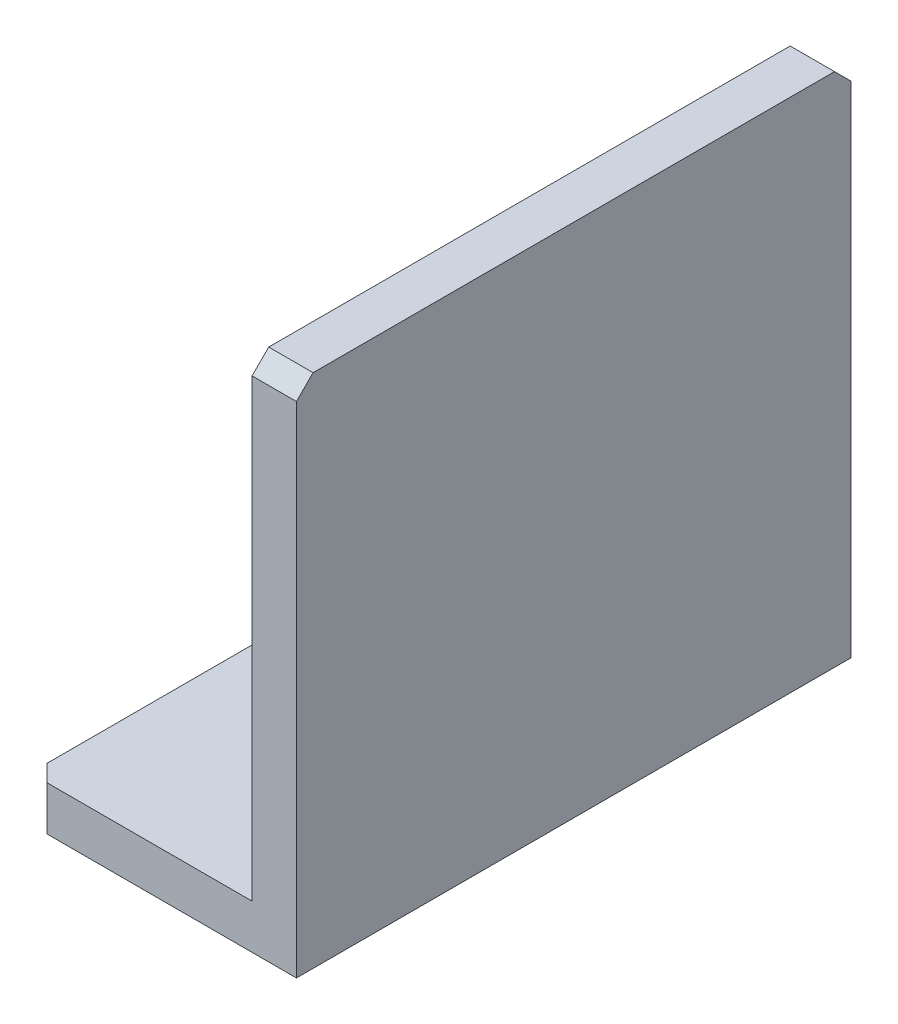
from build123d import *

# Parameters (mm, degrees)
EXTRUDE_1_DEPTH = 50
CHAMFER_1_SIZE  = 3


with BuildPart() as part:
    # 草图2 → 凸台-拉伸1 (new, symmetric)
    with BuildSketch(Plane(origin=(409.637600706, 0.5, -34.379468655), x_dir=(1, 0, 0), z_dir=(0, 0, 1))):
        Polygon((-409.637600706, 92.5), (-409.637600706, -0.5), (-457.637600706, -0.5), (-457.637600706, 7.5), (-417.637600706, 7.5), (-417.637600706, 92.5), align=None)
    extrude(amount=EXTRUDE_1_DEPTH, both=True)

    # 倒角1
    chamfer_1_edges = [part.edges().sort_by_distance(p)[0] for p in [
        (-48, 4, 15.620531345),
        (-4, 93, 15.620531345),
        (-48, 4, -84.379468655),
        (-4, 93, -84.379468655),
    ]]
    chamfer(chamfer_1_edges, length=CHAMFER_1_SIZE)


solid = part.part
